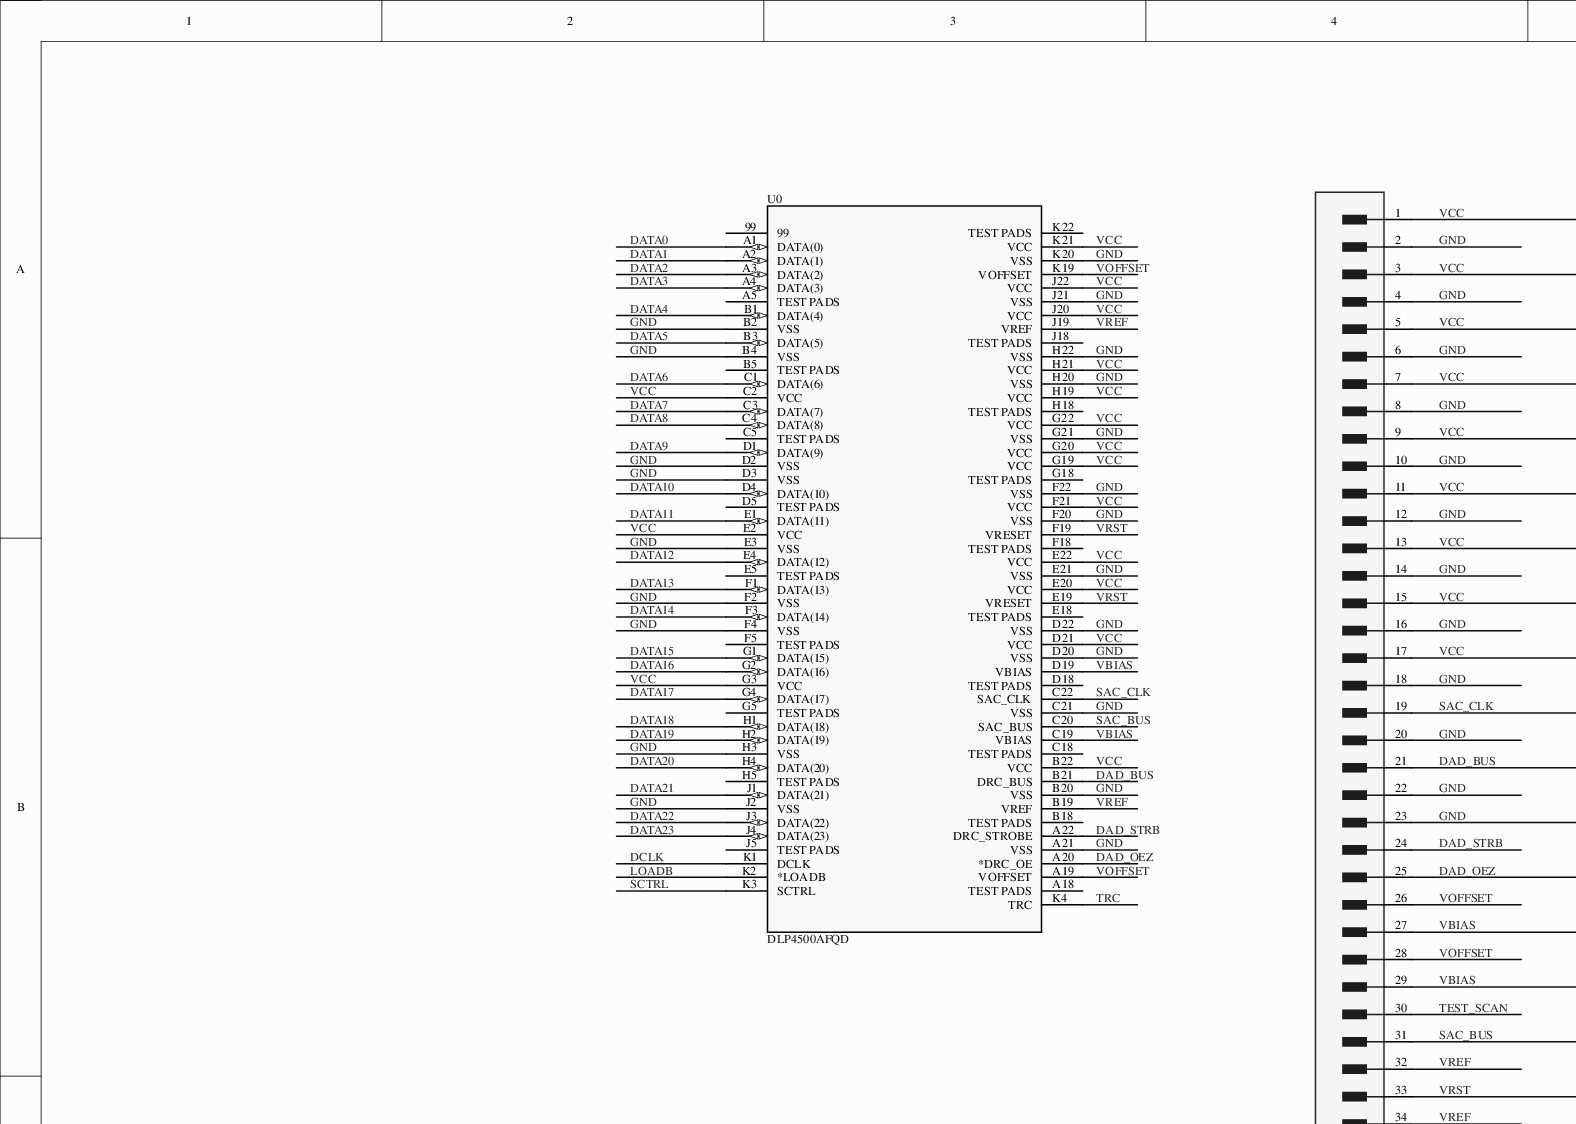
[diagram p0: MISC82783-3.SchDoc, top left]
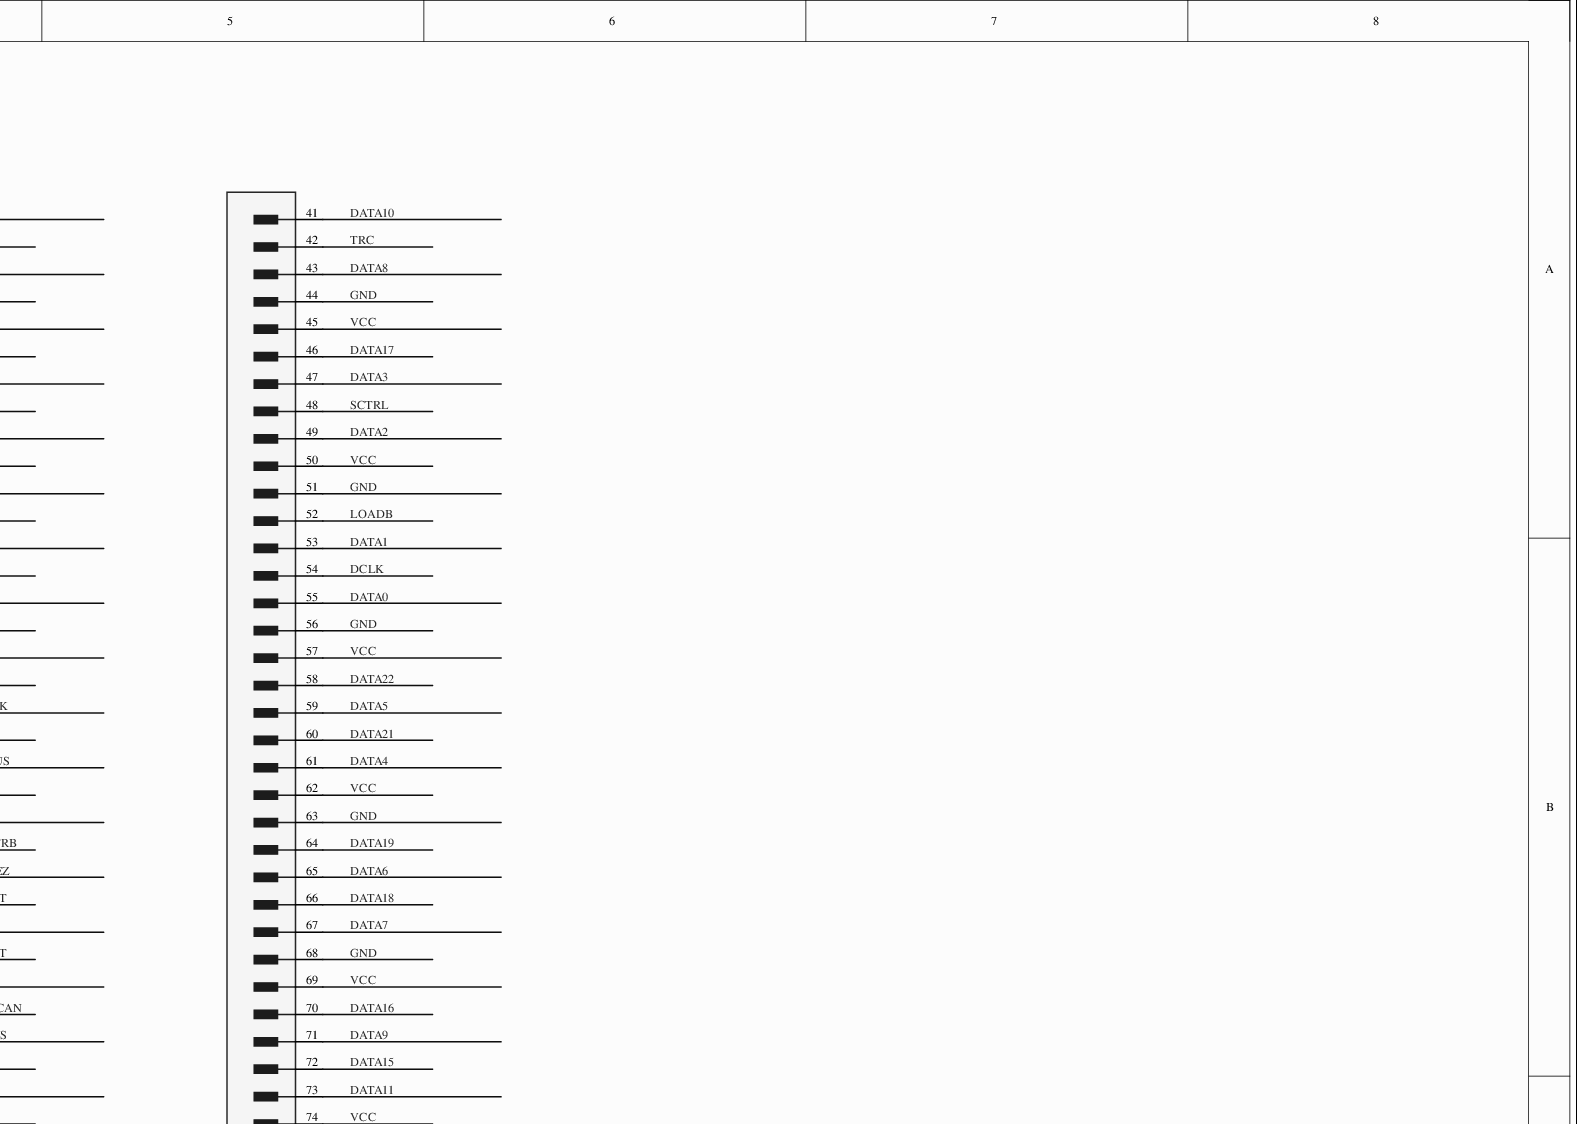
[diagram p1: MISC82783-3.SchDoc, top right]
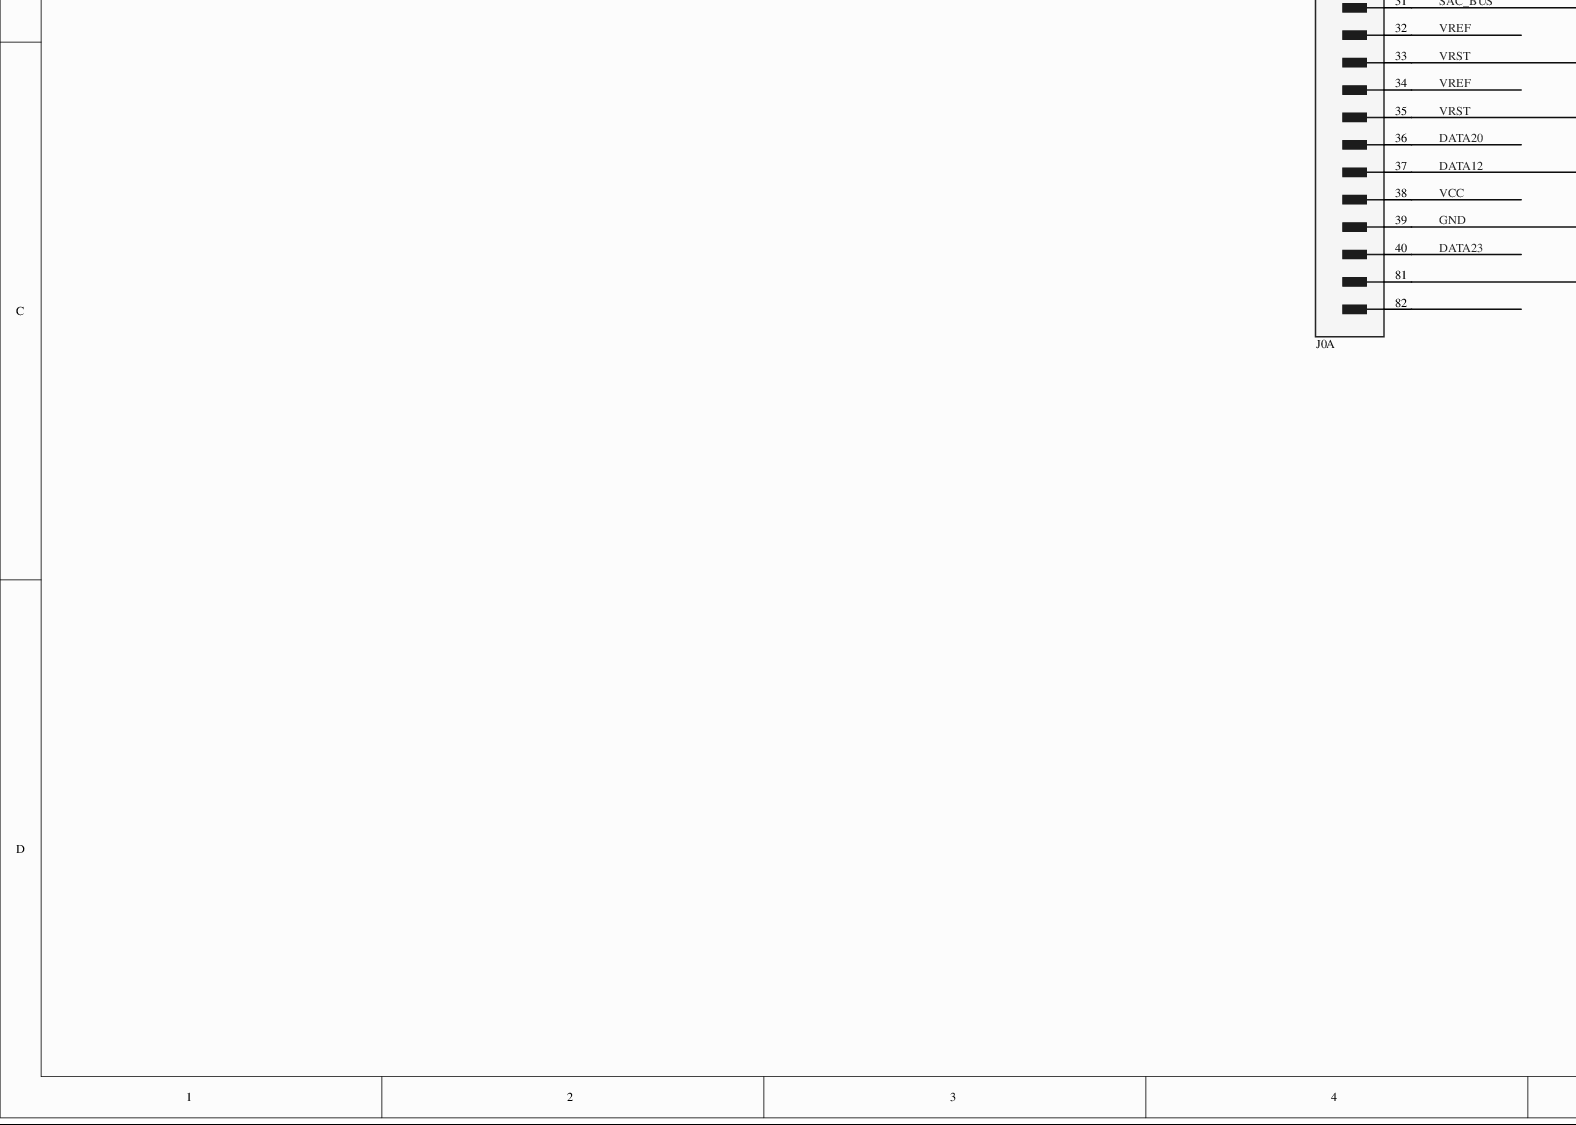
[diagram p2: MISC82783-3.SchDoc, bottom left]
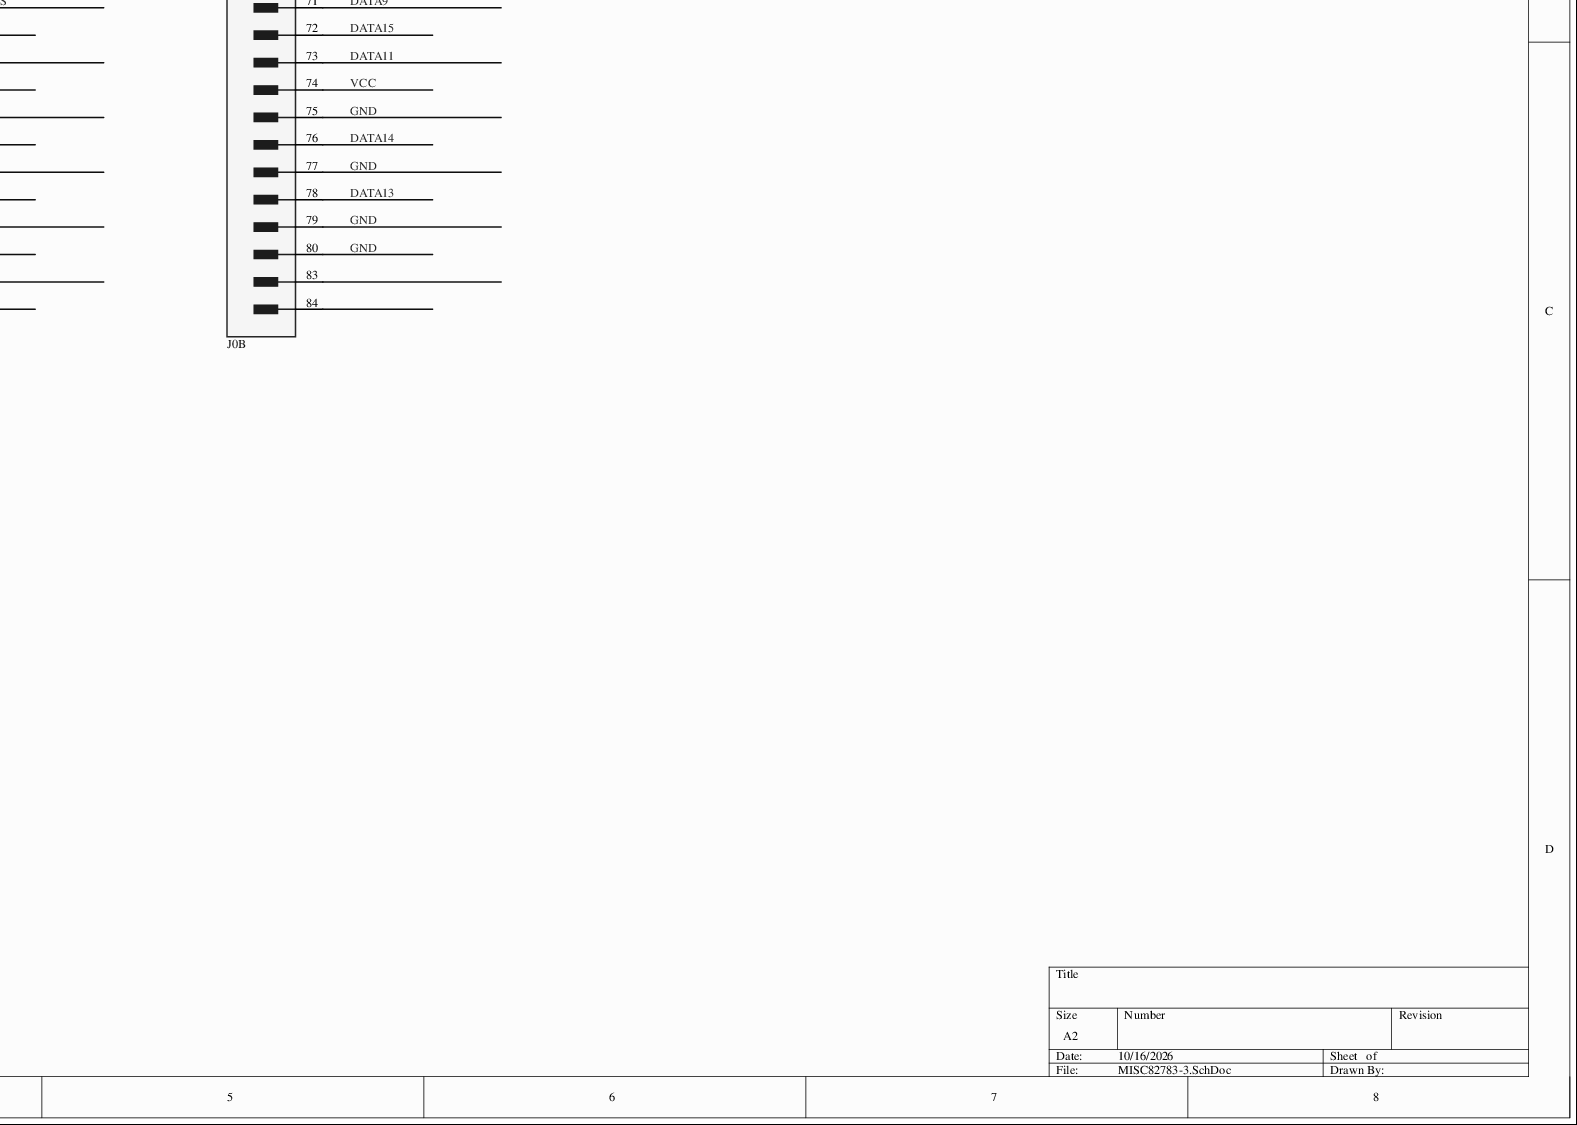
[diagram p3: MISC82783-3.SchDoc, bottom right]
# Altium project MISC82783-2.PrjPcb
1 sheet, 2 parts. Net scope: global (net labels, ports and power ports of the same name join across sheets).
Board file: MISC82783.PcbDoc

## Sheet MISC82783-3.SchDoc
size A2; SheetNumber: 1; SheetTotal: 1

### Parts
J0  DF40C-80DP-0.4V_51  [HIROSE_DF40C-80DP-0.4V_51_0]  (value not drawn)  (parts A,B of 2)
U0  DLP4500AFQD  [LGA_0AFQD_TEX]

### Nets
DAD_BUS: J0.21 U0.B21(DRC_BUS)
DAD_OEZ: J0.25 U0.A20(*DRC_OE)
DAD_STRB: J0.24 U0.A22(DRC_STROBE)
DATA0: J0.55 U0.A1(DATA(0))
DATA1: J0.53 U0.A2(DATA(1))
DATA2: J0.49 U0.A3(DATA(2))
DATA3: J0.47 U0.A4(DATA(3))
DATA4: J0.61 U0.B1(DATA(4))
DATA5: J0.59 U0.B3(DATA(5))
DATA6: J0.65 U0.C1(DATA(6))
DATA7: J0.67 U0.C3(DATA(7))
DATA8: J0.43 U0.C4(DATA(8))
DATA9: J0.71 U0.D1(DATA(9))
DATA10: J0.41 U0.D4(DATA(10))
DATA11: J0.73 U0.E1(DATA(11))
DATA12: J0.37 U0.E4(DATA(12))
DATA13: J0.78 U0.F1(DATA(13))
DATA14: J0.76 U0.F3(DATA(14))
DATA15: J0.72 U0.G1(DATA(15))
DATA16: J0.70 U0.G2(DATA(16))
DATA17: J0.46 U0.G4(DATA(17))
DATA18: J0.66 U0.H1(DATA(18))
DATA19: J0.64 U0.H2(DATA(19))
DATA20: J0.36 U0.H4(DATA(20))
DATA21: J0.60 U0.J1(DATA(21))
DATA22: J0.58 U0.J3(DATA(22))
DATA23: J0.40 U0.J4(DATA(23))
DCLK: J0.54 U0.K1(DCLK)
GND: J0.2 J0.4 J0.6 J0.8 J0.10 J0.12 J0.14 J0.16 J0.18 J0.20 J0.22 J0.23 J0.39 J0.44 J0.51 J0.56 J0.63 J0.68 J0.75 J0.77 J0.79 J0.80 U0.A21(VSS) U0.B2(VSS) U0.B4(VSS) U0.B20(VSS) U0.C21(VSS) U0.D2(VSS) U0.D3(VSS) U0.D20(VSS) U0.D22(VSS) U0.E3(VSS) U0.E21(VSS) U0.F2(VSS) U0.F4(VSS) U0.F20(VSS) U0.F22(VSS) U0.G21(VSS) U0.H3(VSS) U0.H20(VSS) U0.H22(VSS) U0.J2(VSS) U0.J21(VSS) U0.K20(VSS)
LOADB: J0.52 U0.K2(*LOADB)
SAC_BUS: J0.31 U0.C20(SAC_BUS)
SAC_CLK: J0.19 U0.C22(SAC_CLK)
SCTRL: J0.48 U0.K3(SCTRL)
TEST_SCAN: J0.30
TRC: J0.42 U0.K4(TRC)
VBIAS: J0.27 J0.29 U0.C19(VBIAS) U0.D19(VBIAS)
VCC: J0.1 J0.3 J0.5 J0.7 J0.9 J0.11 J0.13 J0.15 J0.17 J0.38 J0.45 J0.50 J0.57 J0.62 J0.69 J0.74 U0.B22(VCC) U0.C2(VCC) U0.D21(VCC) U0.E2(VCC) U0.E20(VCC) U0.E22(VCC) U0.F21(VCC) U0.G3(VCC) U0.G19(VCC) U0.G20(VCC) U0.G22(VCC) U0.H19(VCC) U0.H21(VCC) U0.J20(VCC) U0.J22(VCC) U0.K21(VCC)
VOFFSET: J0.26 J0.28 U0.A19(VOFFSET) U0.K19(VOFFSET)
VREF: J0.32 J0.34 U0.B19(VREF) U0.J19(VREF)
VRST: J0.33 J0.35 U0.E19(VRESET) U0.F19(VRESET)

Not connected (* = marked no-connect by the designer): J0 81(MNT_1) 82(MNT_2) 83(MNT_3) 84(MNT_4); U0 99 A5(TEST_PADS) A18(TEST_PADS) B5(TEST_PADS) B18(TEST_PADS) C5(TEST_PADS) C18(TEST_PADS) D5(TEST_PADS) D18(TEST_PADS) E5(TEST_PADS) E18(TEST_PADS) F5(TEST_PADS) F18(TEST_PADS) G5(TEST_PADS) G18(TEST_PADS) H5(TEST_PADS) H18(TEST_PADS) J5(TEST_PADS) J18(TEST_PADS) K22(TEST_PADS)

### Library data of the parts
U0 = DLP4500AFQD: No Description Available; Mfr_Name: Texas Instruments; RefDes: RefDes; Type: Type